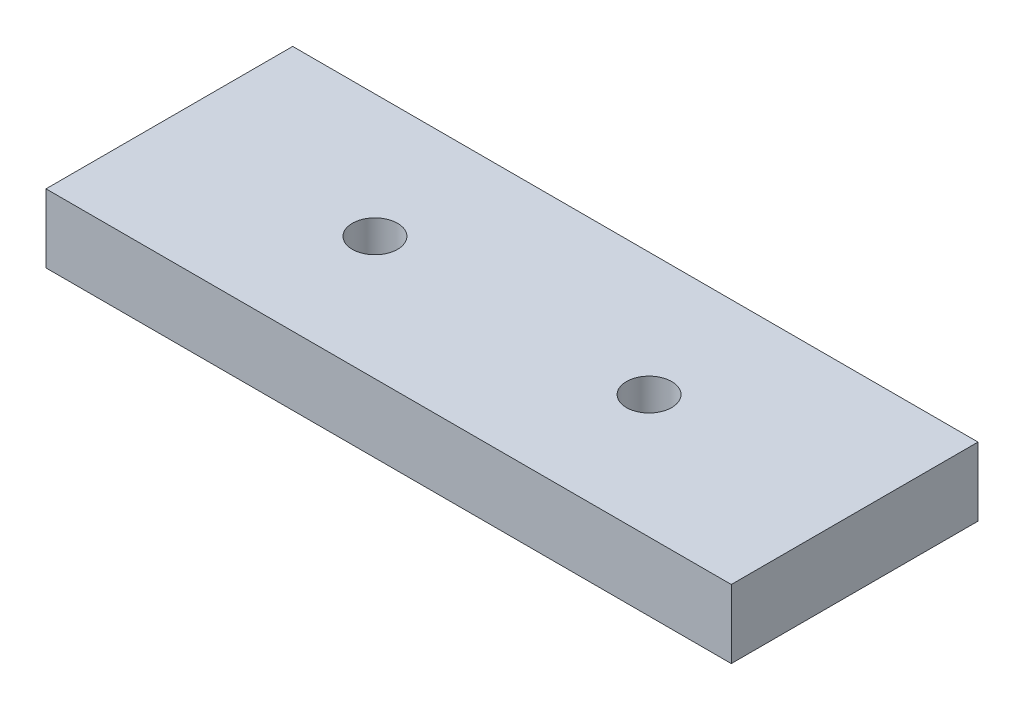
SolidWorks part; units mm, degrees
ref_plane "前视基准面" through (0, 0, 0) normal (0, 0, 1) x (1, 0, 0)
ref_plane "上视基准面" through (0, 0, 0) normal (0, 1, 0) x (1, 0, 0)
ref_plane "右视基准面" through (0, 0, 0) normal (1, 0, 0) x (0, 0, -1)
sketch "草图1" plane through (0, 0, 0) normal (0, 1, 0) x (1, 0, 0)
  line L0 (0, 0) -> (0, -9)
  line L1 (0, -9) -> (50, -9)
  line L2 (50, -9) -> (50, 9)
  line L3 (50, 9) -> (0, 9)
  line L4 (0, 9) -> (0, 0)
  line L5 (0, 0) -> (57.8671, 0) construction
extrude "凸台-拉伸1" add sketch "草图1" along normal mid plane 5
hole_wizard "M4 螺纹孔1" positions "草图3" profile "草图2" tap size "M4" standard "Iso"
sketch "草图3" plane through (0, 2.5, 0) normal (0, 1, 0) x (1, 0, 0)
  line L0 (0, -9) -> (50, -9) construction
  point P0 (15, 0)
  point P2 (35, 0)
  dimension "D1" = 15
  dimension "D2" = 20
  dimension "D3" = 9
  dimension "D4" = 9
cosmetic thread "孔螺蚊线1" parameters "D1"=5, "D2"=4
cosmetic thread "孔螺蚊线2" parameters "D1"=5, "D2"=4
sketch "草图2" plane through (15, 2.5, 0) normal (1, 0, 0) x (0, 0, 1)
  line L0 (0, 0) -> (0, 11.0914)
  line L1 (0, 11.0914) -> (1.65, 10.1)
  line L2 (1.65, 10.1) -> (1.65, 0)
  line L5 (1.65, 0) -> (0, 0)
  line L10 (0, 11.0914) -> (-1.65, 10.1) construction
  line L11 (0, -6.35) -> (0, 107.95) construction
  dimension "螺纹孔钻头直径" = 3.3
  dimension "螺纹孔钻头深度" = 10.1
  dimension "导头角度" = 118
